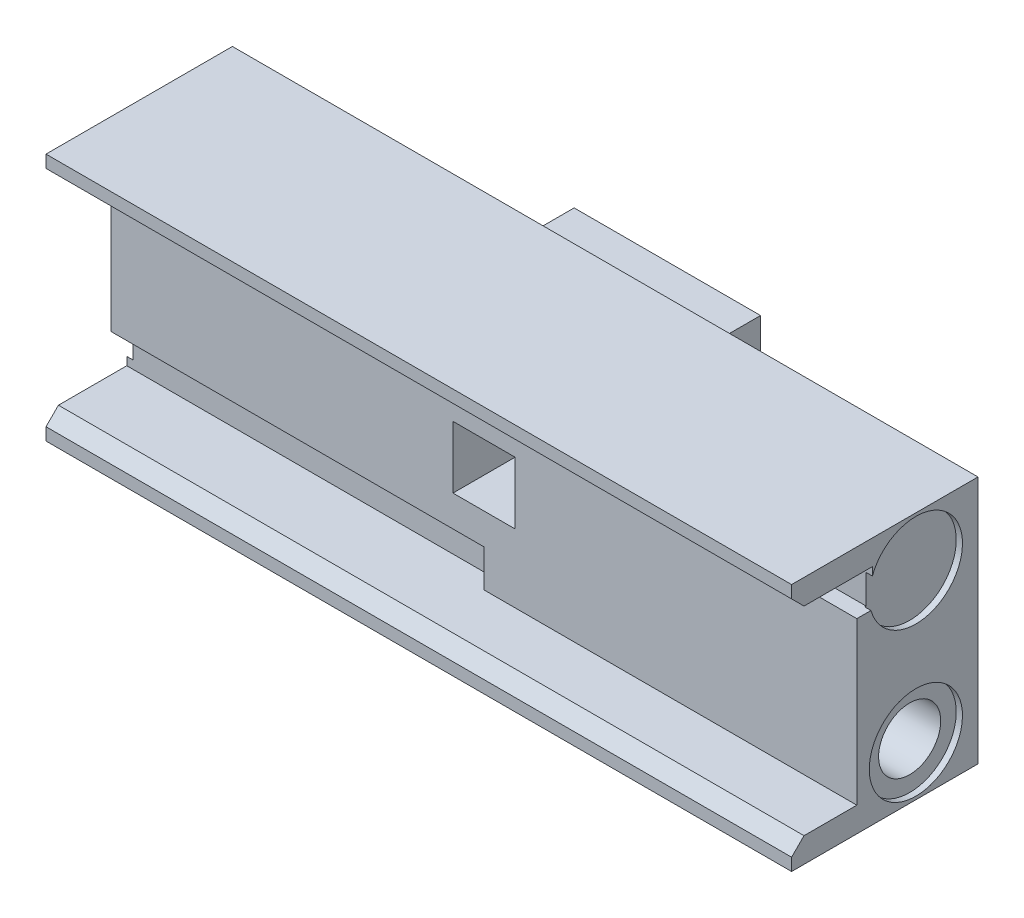
SolidWorks part; units mm, degrees
ref_plane "Front Plane" through (0, 0, 0) normal (0, 0, 1) x (1, 0, 0)
ref_plane "Top Plane" through (0, 0, 0) normal (0, 1, 0) x (1, 0, 0)
ref_plane "Right Plane" through (0, 0, 0) normal (1, 0, 0) x (0, 0, -1)
sketch "Sketch1" plane through (0, 0, 0) normal (0, 0, 1) x (1, 0, 0)
  line L1 (-60, 20) -> (60, 20)
  line L2 (-60, 20) -> (-60, -20)
  line L3 (-60, -20) -> (60, -20)
  line L4 (60, 20) -> (60, -20)
  line L5 (-60, 20) -> (60, -20) construction
  line L6 (-60, -20) -> (60, 20) construction
  point P0 (0, 0)
  dimension "D1" = 120
  dimension "D2" = 40
extrude "Boss-Extrude1" add sketch "Sketch1" along normal blind 30
sketch "Sketch3" plane through (60, 0, 0) normal (1, 0, 0) x (0, 0, -1)
  line L0 (-30, -20) -> (-30, 20) construction
  line L1 (-30, 16) -> (-17, 16)
  line L2 (-30, 16) -> (-30, -16)
  line L3 (-30, -16) -> (-19.5, -16)
  line L4 (-19.5, 10) -> (-19.5, -16)
  line L5 (-30, -20) -> (0, -20) construction
  line L6 (-30, 20) -> (0, 20) construction
  line L8 (-19.5, 10) -> (-17, 10)
  line L9 (-17, 16) -> (-17, 10)
  dimension "D1" = 4
  dimension "D2" = 2.5
  dimension "D3" = 6
  dimension "D4" = 13
  dimension "D5" = 4
extrude "Cut-Extrude1" cut sketch "Sketch3" against normal blind 70
sketch "Sketch4" plane through (-60, 0, 0) normal (-1, 0, 0) x (0, 0, 1)
  line L0 (30, 20) -> (30, -20) construction
  line L1 (30, 16) -> (19.5, 16)
  line L2 (30, 16) -> (30, -16)
  line L3 (30, -16) -> (17, -16)
  line L4 (19.5, 16) -> (19.5, -10)
  line L5 (30, 20) -> (0, 20) construction
  line L7 (30, -20) -> (0, -20) construction
  line L8 (19.5, -10) -> (17, -10)
  line L9 (17, -16) -> (17, -10)
  dimension "D1" = 4
  dimension "D2" = 4
  dimension "D3" = 2.5
  dimension "D4" = 6
  dimension "D5" = 13
extrude "Cut-Extrude2" cut sketch "Sketch4" against normal blind 60
sketch "Sketch5" plane through (0, 0, 0) normal (0, 0, -1) x (-1, 0, 0)
  line L1 (-15, 15) -> (15, 15)
  line L2 (-15, 15) -> (-15, -15)
  line L3 (-15, -15) -> (15, -15)
  line L4 (15, 15) -> (15, -15)
  line L5 (-15, 15) -> (15, -15) construction
  line L6 (-15, -15) -> (15, 15) construction
  point P0 (0, 0)
  dimension "D1" = 30
extrude "Boss-Extrude2" add sketch "Sketch5" along normal blind 10
sketch "Sketch6" plane through (60, 0, 0) normal (1, 0, 0) x (0, 0, -1)
  line L0 (0, 0) -> (-10, 0) construction
  line L1 (-10, 12) -> (-10, -12) construction
  circle A0 centre (-10, 12) radius 7.5
  circle A1 centre (-10, -12) radius 7.5
  dimension "D3" = 15
  dimension "D1" = 10
  dimension "D2" = 24
sketch "Sketch7" plane through (0, 0, 19.5) normal (0, 0, 1) x (1, 0, 0)
  line L1 (-5, 5) -> (5, 5)
  line L2 (-5, 5) -> (-5, -5)
  line L3 (-5, -5) -> (5, -5)
  line L4 (5, 5) -> (5, -5)
  line L5 (-5, 5) -> (5, -5) construction
  line L6 (-5, -5) -> (5, 5) construction
  point P0 (0, 0)
  dimension "D1" = 10
extrude "Cut-Extrude4" cut sketch "Sketch7" against normal blind 10
chamfer "Chamfer1" distance 2 angle 45 2 edges at (0, 16, 30) (0, -16, 30)
extrude "Cut-Extrude5" cut sketch "Sketch6" against normal blind 1
sketch "Sketch9" plane through (59, 0, 0) normal (1, 0, 0) x (0, 0, -1)
  circle A0 centre (-10, -12) radius 5
  dimension "D1" = 10
extrude "Cut-Extrude6" cut sketch "Sketch9" against normal blind 55
mirror "Mirror1" about plane through (0, 0, 0) normal (1, 0, 0) of "Cut-Extrude5"
sketch "Sketch10" plane through (-59, 0, 0) normal (-1, 0, 0) x (0, 0, 1)
  circle A0 centre (10, 12) radius 5
  dimension "D1" = 10
extrude "Cut-Extrude7" cut sketch "Sketch10" against normal blind 55
